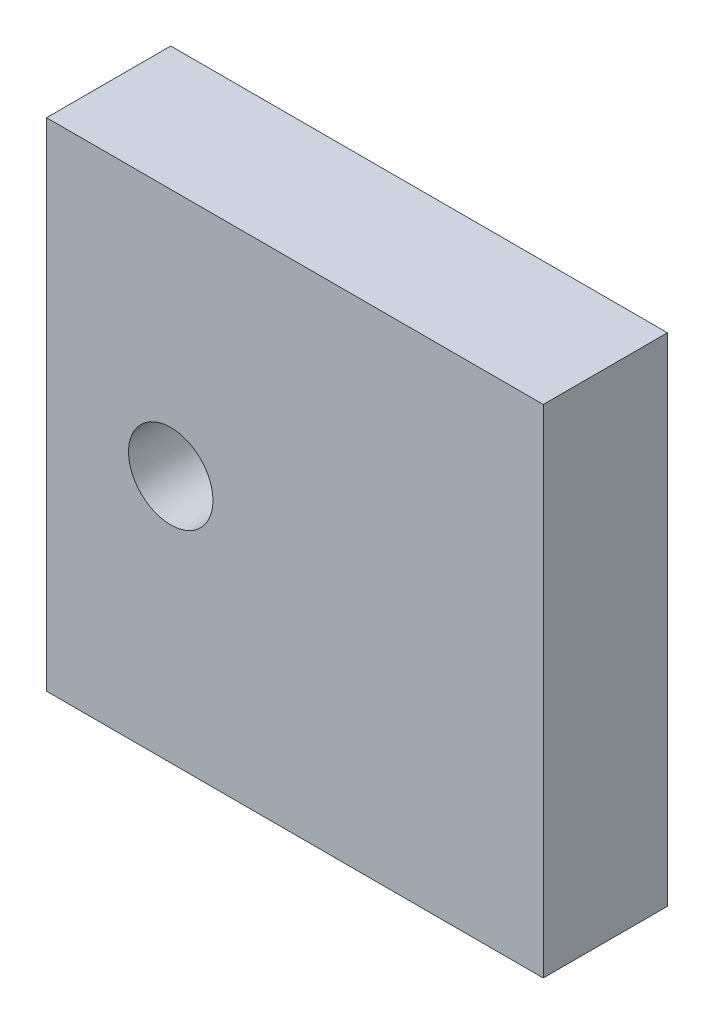
from build123d import *

# Parameters (mm, degrees)
SKETCH_1_W         = 40
SKETCH_1_H         = 40
EXTRUDE_1_DEPTH    = 5
HOLE_WIZARD_M8_1_D = 6.8


with BuildPart() as part:
    # 草图1 → 凸台-拉伸1 (new, symmetric)
    with BuildSketch(Plane.XY):
        Rectangle(SKETCH_1_W, SKETCH_1_H)
    extrude(amount=EXTRUDE_1_DEPTH, both=True)

    # M8 螺纹孔1 (through all)
    with Locations(Plane.XY.offset(5)):
        with Locations((-10, 0)):
            Hole(HOLE_WIZARD_M8_1_D / 2)


solid = part.part
